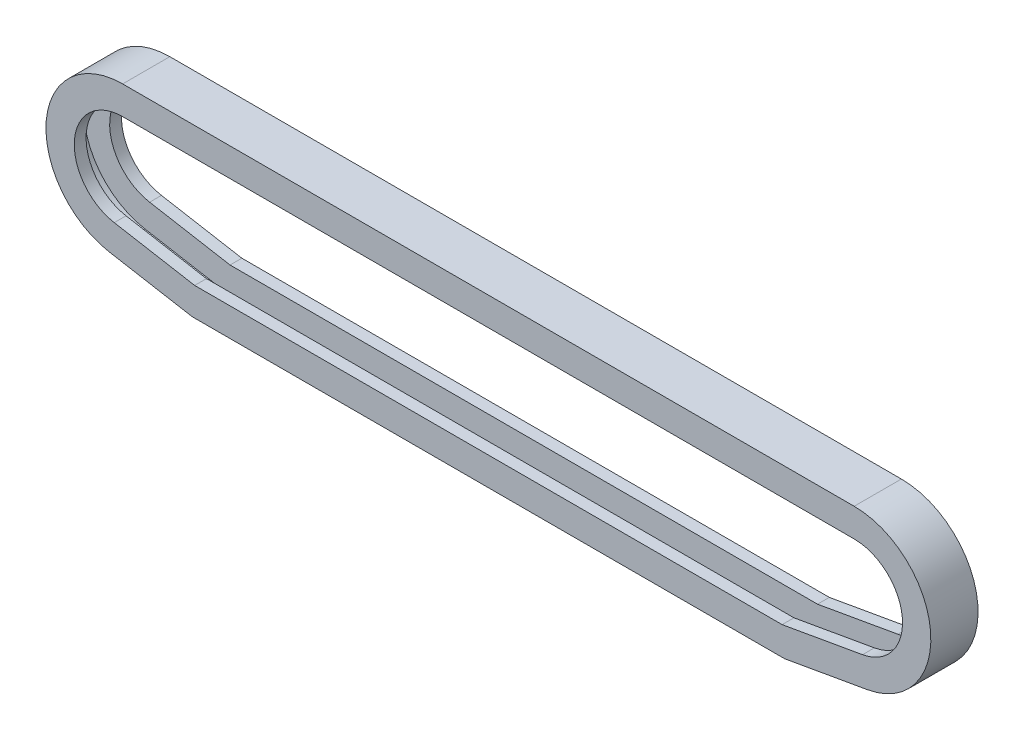
from build123d import *

# Parameters (mm, degrees)
BOSS_EXTRUDE1_DEPTH = 10
CUT_EXTRUDE1_DEPTH  = 5


with BuildPart() as part:
    # Sketch2 → Boss-Extrude1 (new, symmetric)
    with BuildSketch(Plane.XY):
        with BuildLine():
            Line((-155, 32.5), (155, 32.5))
            ThreePointArc((155, 32.5), (187.376327688, 2.832561639), (160.643565774, -32.006251973))
            Line((160.643565774, -32.006251973), (125.524931981, -38.198614636))
            Line((125.524931981, -38.198614636), (-125.524931981, -38.198614636))
            Line((-125.524931981, -38.198614636), (-160.643565774, -32.006251973))
            ThreePointArc((-160.643565774, -32.006251973), (-187.376327688, 2.832561639), (-155, 32.5))
        make_face()
        with BuildLine():
            Line((-155, 20.5), (155, 20.5))
            ThreePointArc((155, 20.5), (175.421991311, 1.786692726), (158.559787642, -20.188558937))
            Line((158.559787642, -20.188558937), (124.475068019, -26.198614636))
            Line((124.475068019, -26.198614636), (-124.475068019, -26.198614636))
            Line((-124.475068019, -26.198614636), (-158.559787642, -20.188558937))
            ThreePointArc((-158.559787642, -20.188558937), (-175.421991311, 1.786692726), (-155, 20.5))
        make_face(mode=Mode.SUBTRACT)
    extrude(amount=BOSS_EXTRUDE1_DEPTH, both=True)

    # Sketch8 → Cut-Extrude1 (cut, symmetric)
    with BuildSketch(Plane.XY):
        with BuildLine():
            Line((125.437443318, -37.198614636), (160.469917597, -31.02144422))
            ThreePointArc((160.469917597, -31.02144422), (186.38013299, 2.745405897), (155, 31.5))
            Line((155, 31.5), (-155, 31.5))
            ThreePointArc((-155, 31.5), (-186.38013299, 2.745405897), (-160.469917597, -31.02144422))
            Line((-160.469917597, -31.02144422), (-125.437443318, -37.198614636))
            Line((-125.437443318, -37.198614636), (125.437443318, -37.198614636))
        make_face()
    extrude(amount=CUT_EXTRUDE1_DEPTH, both=True, mode=Mode.SUBTRACT)


solid = part.part
